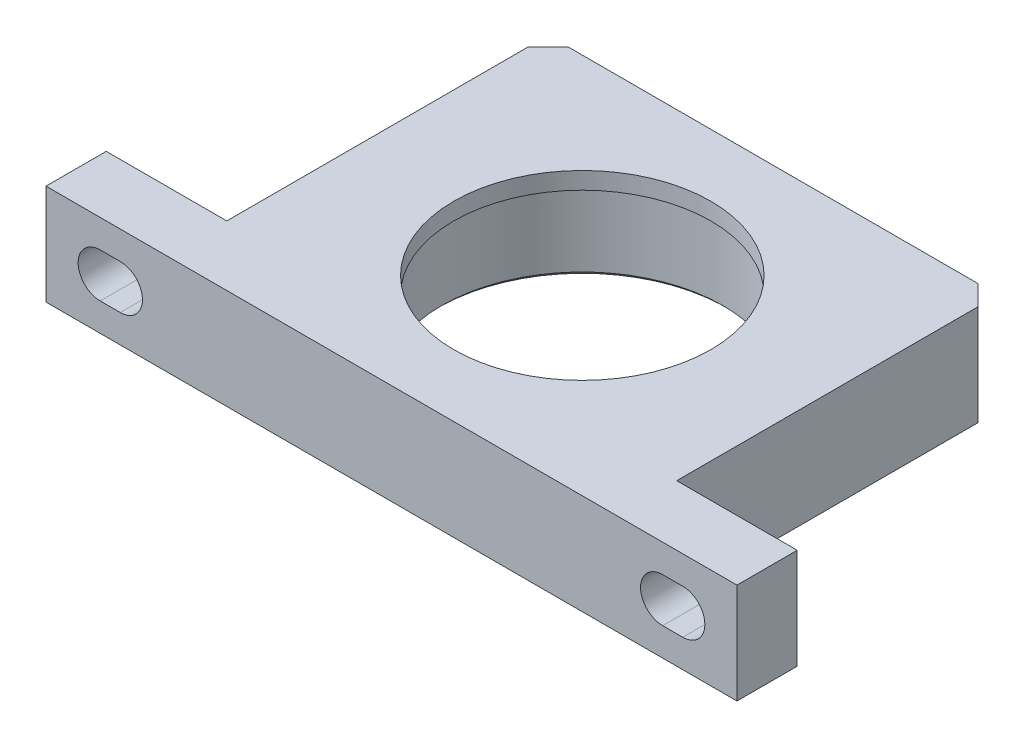
from build123d import *

# Parameters (mm, degrees)
SKETCH1_R           = 64
BOSS_EXTRUDE1_DEPTH = 25
SKETCH2_R           = 70
CUT_EXTRUDE1_DEPTH  = 41.5
CHAMFER1_SIZE       = 2
FILLET1_R           = 2
CUT_EXTRUDE2_DEPTH  = 41.5
BOSS_EXTRUDE2_START = -50
BOSS_EXTRUDE2_DEPTH = 50
CHAMFER2_SIZE       = 10


with BuildPart() as part:
    # Sketch1 → Boss-Extrude1 (new, symmetric)
    with BuildSketch(Plane(origin=(0, 0, 0), x_dir=(1, 0, 0), z_dir=(0, 1, 0))):
        with BuildLine():
            Line((-172, 0), (172, 0))
            Line((172, 0), (172, 30))
            Line((172, 30), (112, 30))
            Line((112, 30), (91.468409221, 116.66864358))
            ThreePointArc((91.468409221, 116.66864358), (0, 189), (-91.468409221, 116.66864358))
            Line((-91.468409221, 116.66864358), (-112, 30))
            Line((-112, 30), (-172, 30))
            Line((-172, 30), (-172, 0))
        make_face()
        with Locations(Location((0, 95, 0), (0, 0, 270))):
            Circle(SKETCH1_R, mode=Mode.SUBTRACT)
    extrude(amount=BOSS_EXTRUDE1_DEPTH, both=True)

    # Sketch2 → Cut-Extrude1 (cut)
    with BuildSketch(Plane.XZ.offset(25)):
        with Locations(Location((0, -95, 0), (0, 0, 270))):
            Circle(SKETCH2_R)
    extrude(amount=-CUT_EXTRUDE1_DEPTH, mode=Mode.SUBTRACT)

    # Chamfer1
    chamfer1_edges = [part.edges().sort_by_distance(p)[0] for p in [
        (0, -25, -25),
    ]]
    chamfer(chamfer1_edges, length=CHAMFER1_SIZE)

    # Fillet1
    fillet1_edges = [part.edges().sort_by_distance(p)[0] for p in [
        (0, 16.5, -25),
    ]]
    fillet(fillet1_edges, radius=FILLET1_R)

    # Sketch3 → Cut-Extrude2 (cut)
    with BuildSketch(Plane(origin=(0, 0, -30), x_dir=(-1, 0, 0), z_dir=(0, 0, -1))):
        with BuildLine():
            Line((135, 11), (145, 11))
            ThreePointArc((145, 11), (156, 0), (145, -11))
            Line((145, -11), (135, -11))
            ThreePointArc((135, -11), (124, 0), (135, 11))
        make_face()
        with BuildLine():
            Line((-145, 11), (-135, 11))
            ThreePointArc((-135, 11), (-124, 0), (-135, -11))
            Line((-135, -11), (-145, -11))
            ThreePointArc((-145, -11), (-156, 0), (-145, 11))
        make_face()
    extrude(amount=-CUT_EXTRUDE2_DEPTH, mode=Mode.SUBTRACT)

    # Sketch4 → Boss-Extrude2 (add)
    with BuildSketch(Plane.XZ.offset(25).offset(BOSS_EXTRUDE2_START)):
        with BuildLine():
            Line((-112, -30), (-112, -190))
            Line((-112, -190), (112, -190))
            Line((112, -190), (112, -30))
            Line((112, -30), (91.468409221, -116.66864358))
            ThreePointArc((91.468409221, -116.66864358), (0, -189), (-91.468409221, -116.66864358))
            Line((-91.468409221, -116.66864358), (-112, -30))
        make_face()
    extrude(amount=BOSS_EXTRUDE2_DEPTH)

    # Chamfer2
    chamfer2_edges = [part.edges().sort_by_distance(p)[0] for p in [
        (112, 0, -190),
        (-112, 0, -190),
    ]]
    chamfer(chamfer2_edges, length=CHAMFER2_SIZE)


solid = part.part
